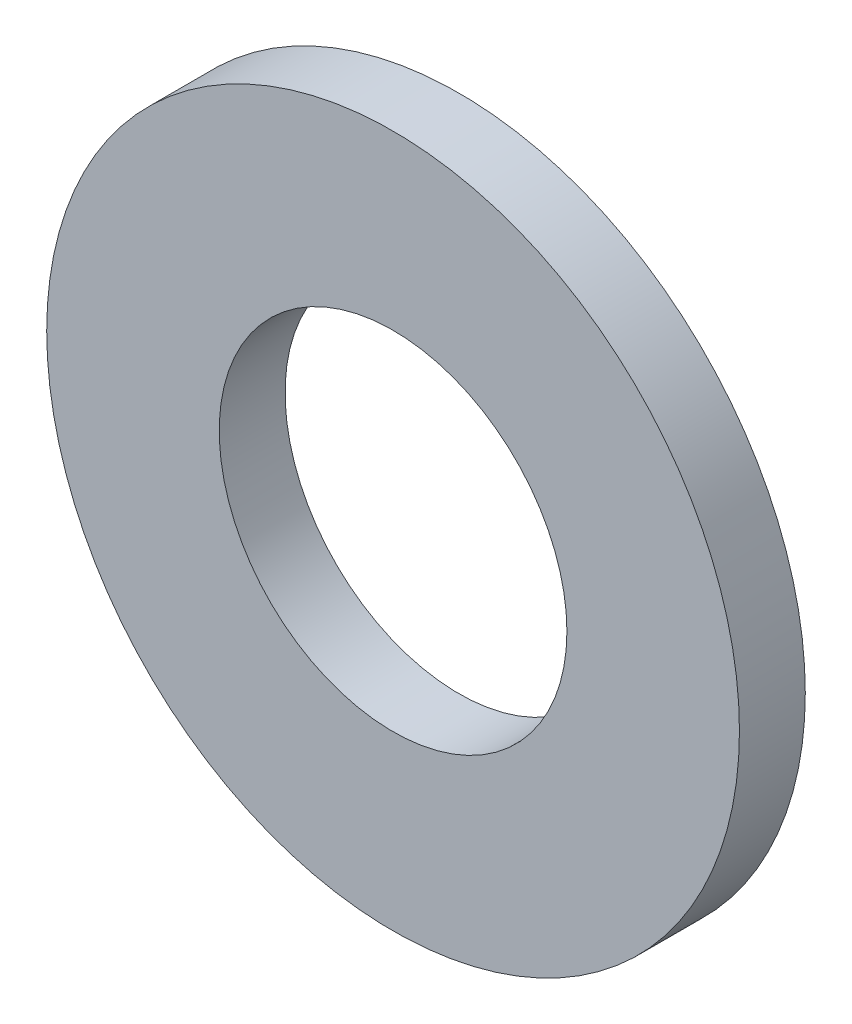
SolidWorks part; units mm, degrees
ref_plane "Front Plane" through (0, 0, 0) normal (0, 0, 1) x (1, 0, 0)
ref_plane "Top Plane" through (0, 0, 0) normal (0, 1, 0) x (1, 0, 0)
ref_plane "Right Plane" through (0, 0, 0) normal (1, 0, 0) x (0, 0, -1)
sketch "Sketch1" plane through (0, 0, 0) normal (0, 0, 1) x (1, 0, 0)
  circle A0 centre (0, 0) radius 13.15
  circle A1 centre (0, 0) radius 6.6
  dimension "D1" = 26.3
  dimension "D2" = 13.2
extrude "Boss-Extrude1" add sketch "Sketch1" along normal mid plane 2.5
